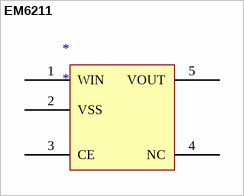
[diagram p0: symbol EM6211]
# Altium schematic symbol library MISC80722-3.SchLib: 1 symbol
Pins are listed as number, name and electrical type; pins without a type are passive.


## EM6211
designator *
pins: 1 WIN, 2 VSS, 3 CE, 4 NC, 5 VOUT